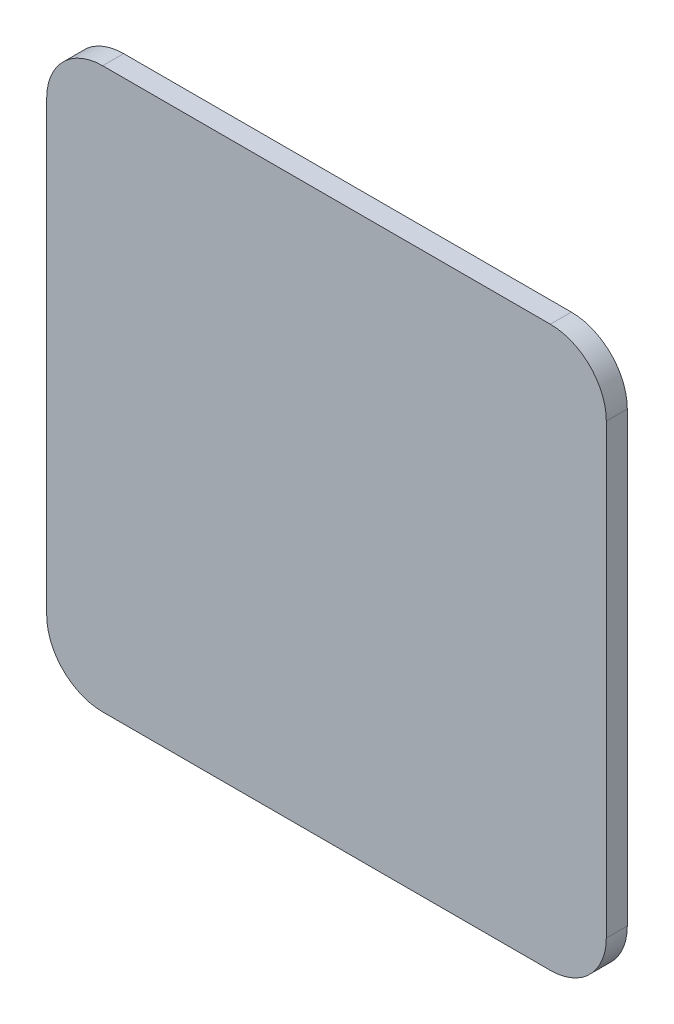
from build123d import *

# Parameters (mm, degrees)
BOSS_EXTRUDE1_DEPTH = 1.5


with BuildPart() as part:
    # Sketch1 → Boss-Extrude1 (new body)
    with BuildSketch(Plane.XY):
        with BuildLine():
            Line((4, 0), (36, 0))
            ThreePointArc((36, 0), (38.828427125, 1.171572875), (40, 4))
            Line((40, 4), (40, 36))
            ThreePointArc((40, 36), (38.828427125, 38.828427125), (36, 40))
            Line((36, 40), (4, 40))
            ThreePointArc((4, 40), (1.171572875, 38.828427125), (0, 36))
            Line((0, 36), (0, 4))
            ThreePointArc((0, 4), (1.171572875, 1.171572875), (4, 0))
        make_face()
    extrude(amount=BOSS_EXTRUDE1_DEPTH)


solid = part.part
